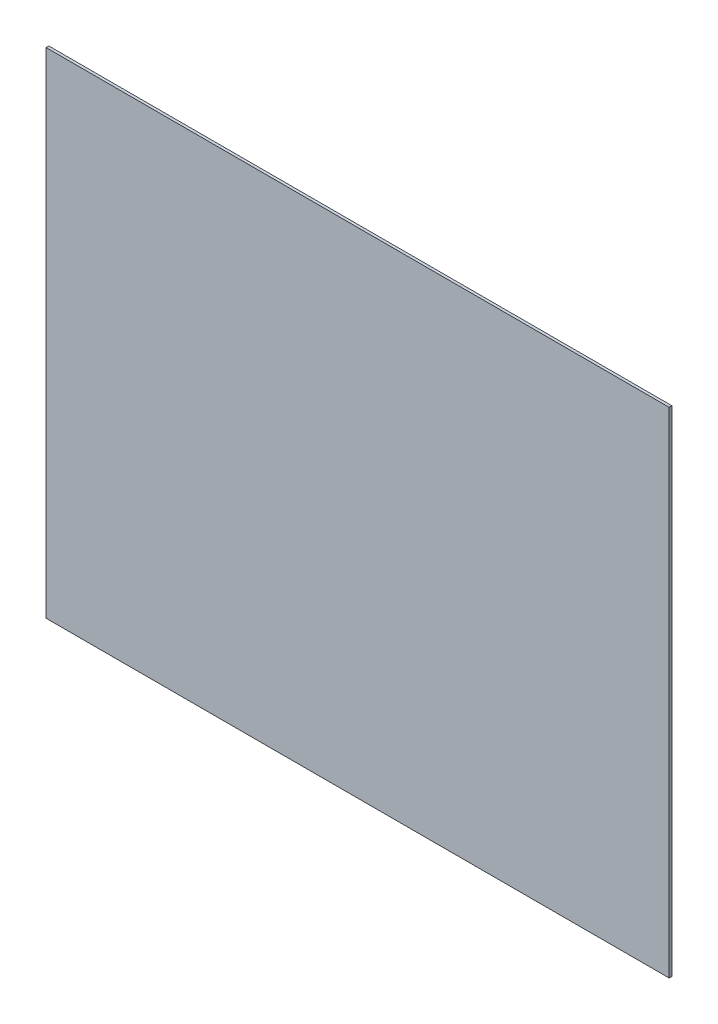
SolidWorks part; units mm, degrees
material "PMMA(有机玻璃)"
ref_plane "前视" through (0, 0, 0) normal (0, 0, 1) x (1, 0, 0)
ref_plane "上视" through (0, 0, 0) normal (0, 1, 0) x (1, 0, 0)
ref_plane "右视" through (0, 0, 0) normal (1, 0, 0) x (0, 0, -1)
sketch "草图1" plane through (0, 0, 0) normal (0, 0, 1) x (1, 0, 0)
  line L1 (-571, 453) -> (571, 453)
  line L2 (-571, 453) -> (-571, -453)
  line L3 (-571, -453) -> (571, -453)
  line L4 (571, 453) -> (571, -453)
  line L5 (-571, 453) -> (571, -453) construction
  line L6 (-571, -453) -> (571, 453) construction
  point P0 (0, 0)
  dimension "D1" = 906
  dimension "D2" = 1142
extrude "凸台-拉伸1" add sketch "草图1" along normal blind 5
hole_wizard "M5 间隙孔1" positions "草图3" profile "草图2" hole size "M5" standard "GB"
sketch "草图3" plane through (0, 0, 5) normal (0, 0, 1) x (1, 0, 0)
  line L0 (-427.5, 273) -> (-427.5, -273) construction
  line L1 (-427.5, -273) -> (427.5, -273) construction
  line L2 (0, 273) -> (0, -273) construction
  line L3 (427.5, 273) -> (-427.5, 273) construction
  line L5 (-427.5, 0) -> (427.5, 0) construction
  line L6 (427.5, -273) -> (427.5, 273) construction
  point P0 (-375, -261)
  point P46 (415.5, 250)
  point P48 (-415.5, 250)
  point P58 (-125, -261)
  point P59 (125, -261)
  point P61 (-125, 261)
  point P62 (125, 261)
  point P64 (-375, 261)
  point P88 (375, -261)
  point P89 (375, 261)
  point P108 (415.5, 0)
  point P109 (-415.5, 0)
  point P110 (415.5, -250)
  point P111 (-415.5, -250)
  dimension "D1" = 12
  dimension "D2" = 12
  dimension "D5" = 3
  dimension "D3" = 12
  dimension "D6" = 4
  dimension "D4" = 2
sketch "草图2" plane through (-375, -261, 5) normal (1, 0, 0) x (0, -1, 0)
  line L0 (0, 0) -> (0, 5)
  line L1 (0, 5) -> (2.75, 5)
  line L2 (2.75, 5) -> (2.75, 0)
  line L5 (2.75, 0) -> (0, 0)
  line L11 (0, -6.35) -> (0, 107.95) construction
  dimension "通孔孔直径" = 5.5
  dimension "通孔孔深度" = 5
